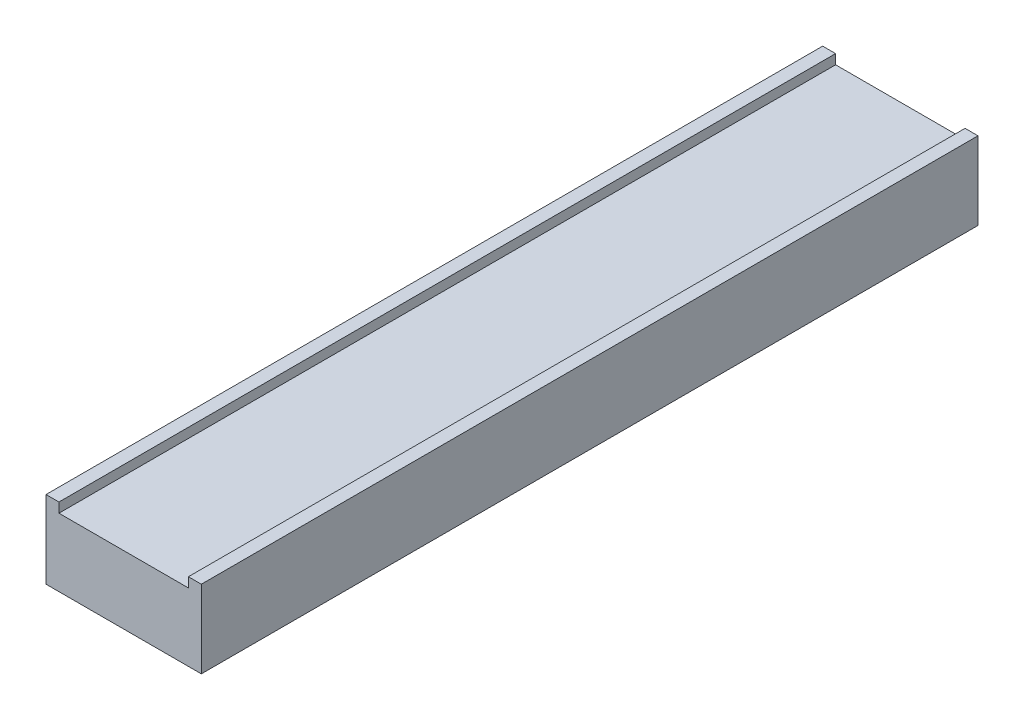
SolidWorks part; units mm, degrees
ref_plane "前视基准面" through (0, 0, 0) normal (0, 0, 1) x (1, 0, 0)
ref_plane "上视基准面" through (0, 0, 0) normal (0, 1, 0) x (1, 0, 0)
ref_plane "右视基准面" through (0, 0, 0) normal (1, 0, 0) x (0, 0, -1)
sketch "草图1" plane through (0, 0, 0) normal (0, 1, 0) x (1, 0, 0)
  line L1 (6, -30) -> (-6, -30)
  line L2 (6, -30) -> (6, 30)
  line L3 (6, 30) -> (-6, 30)
  line L4 (-6, -30) -> (-6, 30)
  line L5 (6, -30) -> (-6, 30) construction
  line L6 (6, 30) -> (-6, -30) construction
  point P0 (0, 0)
  dimension "D1" = 12
  dimension "D2" = 60
extrude "凸台-拉伸1" add sketch "草图1" along normal blind 6
sketch "草图2" plane through (0, 6, 0) normal (0, 1, 0) x (1, 0, 0)
  line L0 (6, 30) -> (-6, 30) construction
  line L1 (5, -30) -> (-5, -30)
  line L2 (5, -30) -> (5, 30)
  line L3 (5, 30) -> (-5, 30)
  line L4 (-5, -30) -> (-5, 30)
  line L5 (5, -30) -> (-5, 30) construction
  line L6 (5, 30) -> (-5, -30) construction
  point P0 (0, 0)
  dimension "D1" = 10
extrude "切除-拉伸1" cut sketch "草图2" against normal blind 0.75
